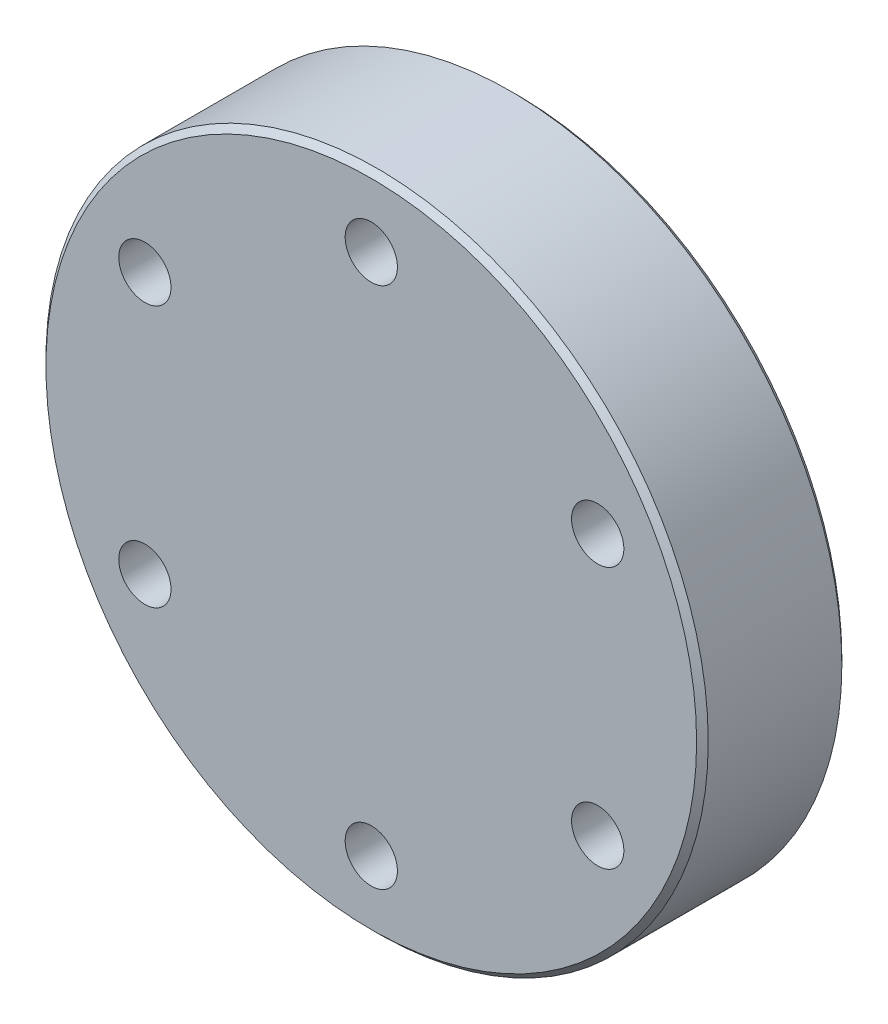
SolidWorks part; units mm, degrees
material "Cr12MoV"
ref_plane "Front Plane" through (0, 0, 0) normal (0, 0, 1) x (1, 0, 0)
ref_plane "Top Plane" through (0, 0, 0) normal (0, 1, 0) x (1, 0, 0)
ref_plane "Right Plane" through (0, 0, 0) normal (1, 0, 0) x (0, 0, -1)
sketch "Sketch1" plane through (0, 0, 0) normal (0, 0, 1) x (1, 0, 0)
  circle A0 centre (0, 0) radius 57
  dimension "D1" = 114
extrude "Boss-Extrude1" add sketch "Sketch1" along normal blind 25
chamfer "Chamfer3" distance 1 angle 45 2 edges at (57, 0, 0) (57, 0, 25)
hole_wizard "Hole size (per socket head cap screw type)1" positions "Sketch2" profile "Sketch3" counterbore size "M8" standard "GB" end condition through all
sketch "Sketch2" plane through (0, 0, 0) normal (0, 0, -1) x (-1, 0, 0)
  line L0 (0, 0) -> (0, 45)
  circle A0 centre (0, 0) radius 45
  point P0 (0, 45)
  dimension "D1" = 90
sketch "Sketch3" plane through (0, 45, 0) normal (1, 0, 0) x (0, 1, 0)
  line L0 (0, 0) -> (0, 25)
  line L1 (0, 25) -> (4.5, 25)
  line L3 (4.5, 25) -> (4.5, 12)
  line L4 (4.5, 12) -> (7.5, 12)
  line L5 (7.5, 12) -> (7.5, 0)
  line L7 (7.5, 0) -> (0, 0)
  line L11 (0, -6.35) -> (0, 107.95) construction
  dimension "通孔孔直径" = 9
  dimension "通孔孔深度" = 25
  dimension "柱形沉头孔直径" = 15
  dimension "柱形沉头孔深度" = 12
pattern_circular "CirPattern1" count 6 over 360 about axis through (0, 0, 0) along (0, 0, 1) of "Hole size (per socket head cap screw type)1"
